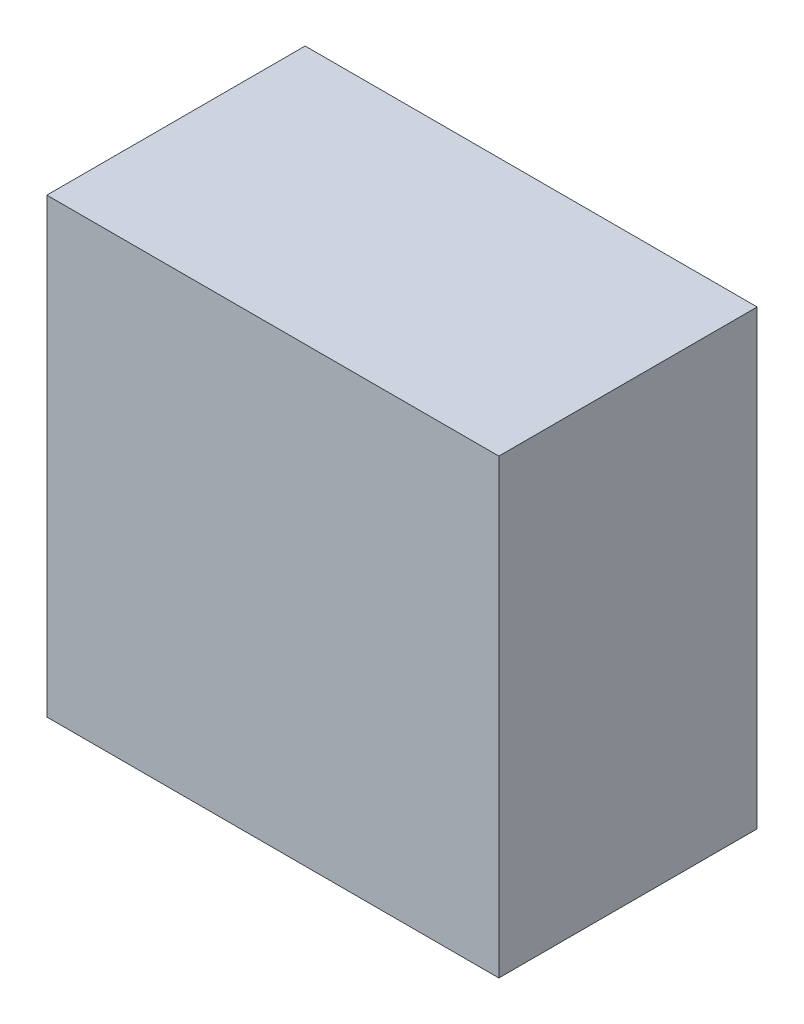
SolidWorks part; units mm, degrees
ref_plane "Front Plane" through (0, 0, 0) normal (0, 0, 1) x (1, 0, 0)
ref_plane "Top Plane" through (0, 0, 0) normal (0, 1, 0) x (1, 0, 0)
ref_plane "Right Plane" through (0, 0, 0) normal (1, 0, 0) x (0, 0, -1)
sketch "Sketch1" plane through (0, 0, 0) normal (0, 0, 1) x (1, 0, 0)
  line L0 (-109, -39) -> (-74, -39) construction
  line L1 (-74, -39) -> (-74, -4) construction
  line L2 (-74, -4) -> (-109, -4) construction
  line L3 (-109, -4) -> (-109, -39) construction
  line L4 (-109, -39) -> (-74, -39)
  line L5 (-74, -39) -> (-74, -4)
  line L6 (-74, -4) -> (-109, -4)
  line L7 (-109, -4) -> (-109, -39)
extrude "Boss-Extrude1" add sketch "Sketch1" against normal blind 20
shell "Shell1" thickness 1
